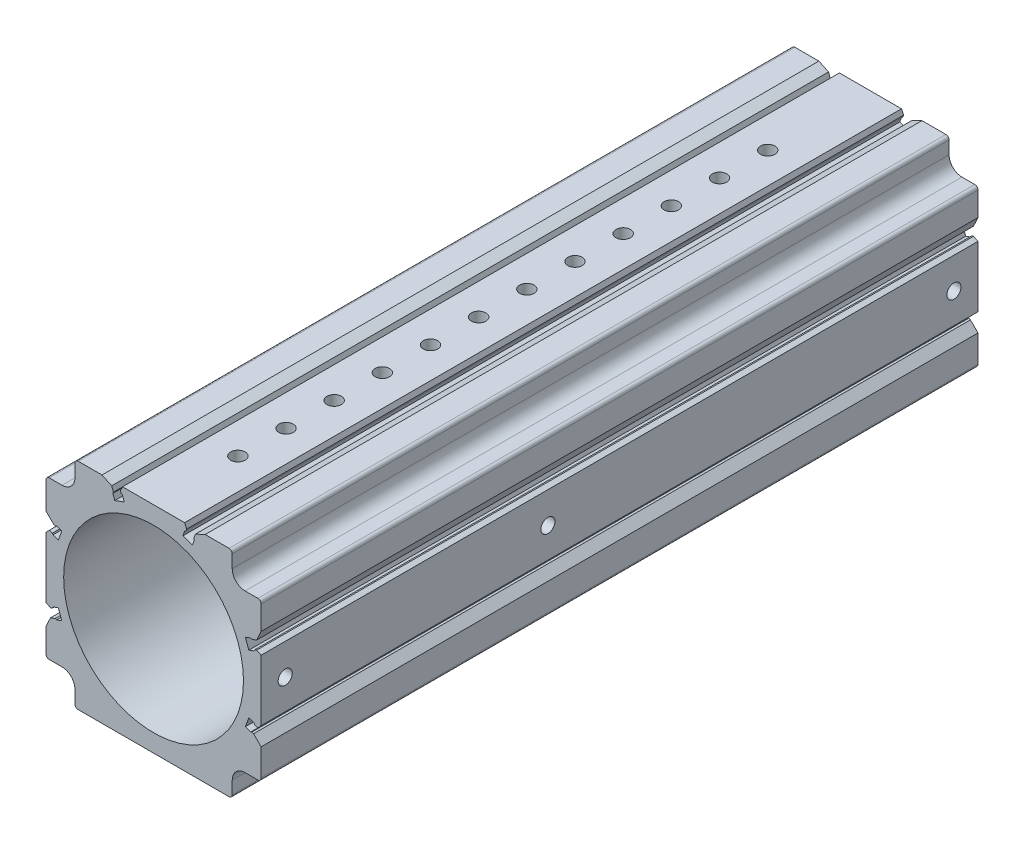
SolidWorks part; units mm, degrees
material "电镀钢"
ref_plane "Front Plane" through (0, 0, 0) normal (0, 0, 1) x (1, 0, 0)
ref_plane "Top Plane" through (0, 0, 0) normal (0, 1, 0) x (1, 0, 0)
ref_plane "Right Plane" through (0, 0, 0) normal (1, 0, 0) x (0, 0, -1)
sketch "Sketch1" plane through (0, 0, 0) normal (0, 0, 1) x (1, 0, 0)
  line L0 (-44.8, 67) -> (-36.9132, 67)
  line L1 (36.9132, 67) -> (44.8, 67)
  line L2 (67, 36.9132) -> (67, 44.8)
  line L3 (67, -44.8) -> (67, -36.9132)
  line L4 (-44.8, -67) -> (-36.9132, -67)
  line L5 (36.9132, -67) -> (44.8, -67)
  line L6 (-67, -44.8) -> (-67, -36.9132)
  line L7 (-67, 44.8) -> (-67, 36.9132)
  line L77 (67, -32.6) -> (67, -36.9132)
  line L79 (67, 27.5) -> (66.1, 27.5)
  line L80 (67, 57) -> (67, 44.8)
  line L81 (66.1, 32.6) -> (67, 32.6)
  line L82 (67, 27.5) -> (67, -27.5)
  line L83 (66.1, -27.5) -> (67, -27.5)
  line L84 (67, -32.6) -> (66.1, -32.6)
  line L85 (67, 36.9132) -> (67, 32.6)
  line L86 (65.5, -26.9) -> (62, -26.9)
  line L87 (62, 26.9) -> (65.5, 26.9)
  line L88 (62, -33.2) -> (65.5, -33.2)
  line L89 (65.5, 33.2) -> (62, 33.2)
  line L90 (62, -26.9) -> (62, -33.2)
  line L91 (62, 33.2) -> (62, 26.9)
  line L92 (57, -67) -> (44.8, -67)
  line L94 (67, -44.8) -> (67, -57)
  line L98 (44.8, 67) -> (57, 67)
  line L99 (32.6, 67) -> (36.9132, 67)
  line L100 (-36.9132, -67) -> (36.9132, -67)
  line L101 (33.2, 62) -> (33.2, 65.5)
  line L102 (26.9, 62) -> (33.2, 62)
  line L105 (32.6, 67) -> (32.6, 66.1)
  line L106 (27.5, 66.1) -> (27.5, 67)
  line L107 (-27.5, 67) -> (27.5, 67)
  line L108 (26.9, 65.5) -> (26.9, 62)
  line L109 (-33.2, 62) -> (-26.9, 62)
  line L110 (-26.9, 62) -> (-26.9, 65.5)
  line L111 (-27.5, 67) -> (-27.5, 66.1)
  line L112 (-36.9132, 67) -> (-32.6, 67)
  line L113 (-32.6, 66.1) -> (-32.6, 67)
  line L114 (-33.2, 65.5) -> (-33.2, 62)
  line L116 (-44.8, -67) -> (-57, -67)
  line L120 (-57, 67) -> (-44.8, 67)
  line L122 (-67, 32.6) -> (-67, 36.9132)
  line L123 (-62, 26.9) -> (-62, 33.2)
  line L124 (-65.5, 26.9) -> (-62, 26.9)
  line L125 (-62, 33.2) -> (-65.5, 33.2)
  line L126 (-62, -33.2) -> (-62, -26.9)
  line L127 (-62, -26.9) -> (-65.5, -26.9)
  line L128 (-65.5, -33.2) -> (-62, -33.2)
  line L130 (-67, 32.6) -> (-66.1, 32.6)
  line L131 (-67, -27.5) -> (-66.1, -27.5)
  line L132 (-66.1, 27.5) -> (-67, 27.5)
  line L133 (-66.1, -32.6) -> (-67, -32.6)
  line L134 (-67, -57) -> (-67, -44.8)
  line L135 (-67, -36.9132) -> (-67, -32.6)
  line L136 (-67, -27.5) -> (-67, 27.5)
  line L139 (-67, 44.8) -> (-67, 57)
  line L140 (-65.5, 33.2) -> (-66.1, 32.6)
  line L141 (-66.1, 27.5) -> (-65.5, 26.9)
  line L142 (-65.5, -26.9) -> (-66.1, -27.5)
  line L143 (-66.1, -32.6) -> (-65.5, -33.2)
  line L144 (65.5, -33.2) -> (66.1, -32.6)
  line L145 (66.1, -27.5) -> (65.5, -26.9)
  line L146 (65.5, 26.9) -> (66.1, 27.5)
  line L147 (66.1, 32.6) -> (65.5, 33.2)
  line L148 (33.2, 65.5) -> (32.6, 66.1)
  line L149 (27.5, 66.1) -> (26.9, 65.5)
  line L150 (-26.9, 65.5) -> (-27.5, 66.1)
  line L151 (-32.6, 66.1) -> (-33.2, 65.5)
  arc A15 (-67, -57) -> (-57, -67) centre (-57, -57) ccw
  arc A18 (57, -67) -> (67, -57) centre (57, -57) ccw
  arc A21 (67, 57) -> (57, 67) centre (57, 57) ccw
  arc A24 (-57, 67) -> (-67, 57) centre (-57, 57) ccw
  circle A25 centre (0, 0) radius 56
extrude "Boss-Extrude1" add sketch "Sketch1" along normal blind 446.5
sketch "Sketch3" plane through (0, 0, 446.5) normal (0, 0, 1) x (1, 0, 0)
  line L1 (-49, 49) -> (-73.0007, 49)
  line L2 (-49, 49) -> (-49, 80.3117)
  line L3 (-49, 80.3117) -> (-73.0007, 80.3117)
  line L4 (-73.0007, 49) -> (-73.0007, 80.3117)
  line L5 (-49, 49) -> (-73.0007, 80.3117) construction
  line L6 (-49, 80.3117) -> (-73.0007, 49) construction
  line L8 (-32.6, 67) -> (-57, 67) construction
  line L9 (-67, 57) -> (-67, 32.6) construction
  point P0 (-61.0004, 64.6558)
  dimension "D1" = 18
  dimension "D2" = 18
extrude "Cut-Extrude2" cut sketch "Sketch3" against normal through all
fillet "Fillet1" radius 8 1 edges at (-49, 49, 223.25)
pattern_circular "CirPattern1" count 4 over 360 about axis through (0, 0, 0) along (0, 0, 1) of "Cut-Extrude2", "Fillet1"
hole_wizard "Ø9.0 (9) Diameter Hole1" positions "Sketch6" profile "Sketch8" hole size "Ø9.0" standard "GB"
sketch "Sketch6" plane through (0, 67, 0) normal (0, -1, 0) x (-1, 0, 0)
  line L0 (0, 0) -> (0, -285.4047) construction
  line L4 (49, -446.5) -> (-49, -446.5) construction
  point P0 (0, -394)
  dimension "D1" = 52.5
sketch "Sketch8" plane through (0, 67, 394) normal (1, 0, 0) x (0, 0, 1)
  line L0 (0, 0) -> (0, 22.7039)
  line L1 (0, 22.7039) -> (4.5, 20)
  line L2 (4.5, 20) -> (4.5, 0)
  line L5 (4.5, 0) -> (0, 0)
  line L10 (0, 22.7039) -> (-4.5, 20) construction
  line L11 (0, -6.35) -> (0, 107.95) construction
  dimension "孔直径" = 9
  dimension "孔深度" = 20
  dimension "导头角度" = 118
hole_wizard "M12 Tapped Hole1" positions "Sketch9" profile "Sketch11" tap size "M12" standard "GB"
sketch "Sketch9" plane through (67, -134, 0) normal (-1, 0, 0) x (0, 0, -1)
  line L0 (0, -134) -> (-113.15, -134) construction
  line L4 (-411, -106.5) -> (-411, -161.5) construction
  point P2 (-394, -134)
  dimension "D1" = 17
sketch "Sketch11" plane through (67, 0, 394) normal (0, 1, 0) x (0, 0, -1)
  line L0 (0, 0) -> (0, 32.3144)
  line L1 (0, 32.3144) -> (5.1, 29.25)
  line L2 (5.1, 29.25) -> (5.1, 0)
  line L5 (5.1, 0) -> (0, 0)
  line L10 (0, 32.3144) -> (-5.1, 29.25) construction
  line L11 (0, -6.35) -> (0, 107.95) construction
  dimension "螺纹孔钻头直径" = 10.2
  dimension "螺纹孔钻头深度" = 29.25
  dimension "导头角度" = 118
cosmetic thread "Cosmetic thread 4" [suppressed] parameters "D1"=4.7084, "D2"=12
hole_wizard "M12 Tapped Hole2" positions "Sketch16" profile "Sketch17" tap size "M12" standard "GB"
sketch "Sketch16" plane through (67, 0, 0) normal (-1, 0, 0) x (0, 0, 1)
  point P0 (17, 0)
  dimension "D1" = 17
sketch "Sketch17" plane through (67, 0, 17) normal (0, 1, 0) x (0, 0, -1)
  line L0 (0, 0) -> (0, 32.3144)
  line L1 (0, 32.3144) -> (5.1, 29.25)
  line L2 (5.1, 29.25) -> (5.1, 0)
  line L5 (5.1, 0) -> (0, 0)
  line L10 (0, 32.3144) -> (-5.1, 29.25) construction
  line L11 (0, -6.35) -> (0, 107.95) construction
  dimension "螺纹孔钻头直径" = 10.2
  dimension "螺纹孔钻头深度" = 29.25
  dimension "导头角度" = 118
cosmetic thread "Cosmetic thread 5" [suppressed] parameters "D1"=4.7084, "D2"=12
pattern_linear "LPattern1" count 12 spacing 30 along (0, 0, -1) of "Ø9.0 (9) Diameter Hole1"
hole_wizard "G1/8 Tapped Hole1" positions "Sketch18" profile "Sketch19" tap size "G1/8" standard "GB"
sketch "Sketch18" plane through (67, 0, 0) normal (1, 0, 0) x (0, 0, -1)
  line L1 (0, -27.5) -> (0, 27.5) construction
  point P0 (-267.9, 0)
  dimension "D1" = 267.9
sketch "Sketch19" plane through (67, 0, 267.9) normal (0, 1, 0) x (0, 0, -1)
  line L0 (0, 0) -> (0, 24.8238)
  line L1 (0, 24.8238) -> (4.4, 22.18)
  line L2 (4.4, 22.18) -> (4.4, 0)
  line L5 (4.4, 0) -> (0, 0)
  line L10 (0, 24.8238) -> (-4.4, 22.18) construction
  line L11 (0, -6.35) -> (0, 107.95) construction
  dimension "螺纹孔钻头直径" = 8.8
  dimension "螺纹孔钻头深度" = 22.18
  dimension "导头角度" = 118
cosmetic thread "Cosmetic thread 9" parameters "D1"=4.6551, "D2"=9.728
fillet "Fillet2" radius 2 8 edges at (49, 67, 223.25) (67, 49, 223.25) (67, -49, 223.25) (49, -67, 223.25) (-49, -67, 223.25) (-67, -49, 223.25) (-67, 49, 223.25) (-49, 67, 223.25)
sketch "Sketch20" plane through (67, 0, 0) normal (1, 0, 0) x (0, 0, -1)
  line L0 (-431.5, 0) -> (-15, 0) construction
  line L1 (-446.5, -27.5) -> (-446.5, 27.5) construction
  line L2 (0, -27.5) -> (0, 27.5) construction
  circle A0 centre (-431.5, 0) radius 5
  circle A1 centre (-15, 0) radius 5
  dimension "D1" = 15
  dimension "D2" = 15
hole_wizard "G1/8 Tapped Hole2" positions "Sketch21" profile "Sketch22" tap size "G1/8" standard "GB"
sketch "Sketch21" plane through (67, 0, 0) normal (1, 0, 0) x (0, 0, -1)
  point P0 (-431.5, 0)
  point P3 (-15, 0)
sketch "Sketch22" plane through (67, 0, 431.5) normal (0, 1, 0) x (0, 0, -1)
  line L0 (0, 0) -> (0, 24.8238)
  line L1 (0, 24.8238) -> (4.4, 22.18)
  line L2 (4.4, 22.18) -> (4.4, 0)
  line L5 (4.4, 0) -> (0, 0)
  line L10 (0, 24.8238) -> (-4.4, 22.18) construction
  line L11 (0, -6.35) -> (0, 107.95) construction
  dimension "螺纹孔钻头直径" = 8.8
  dimension "螺纹孔钻头深度" = 22.18
  dimension "导头角度" = 118
cosmetic thread "Cosmetic thread 10" parameters "D1"=4.6551, "D2"=9.728
cosmetic thread "Cosmetic thread 11" parameters "D1"=4.6551, "D2"=9.728
sketch "Sketch23" plane through (0, 0, 0) normal (0, 0, -1) x (-1, 0, 0)
  line L0 (-23.1301, -51) -> (23.1301, -51)
  line L1 (47, -67) -> (-47, -67) construction
  circle A0 centre (0, 0) radius 56 construction
  arc A1 (-23.1301, -51) -> (23.1301, -51) centre (0, 0) ccw
  dimension "D1" = 16
extrude "Boss-Extrude2" [suppressed] add sketch "Sketch23" against normal through all
fillet "Fillet3" [suppressed] radius 10
other "Move Face1" [suppressed] parameters "D1"=6.5
sketch "Sketch24" plane through (0, 67, 0) normal (0, 1, 0) x (1, 0, 0)
  circle A0 centre (0, -394) radius 8
  dimension "D1" = 16
extrude "Cut-Extrude3" [suppressed] cut sketch "Sketch24" against normal blind 4
pattern_linear "LPattern2" [suppressed] count 7 spacing 30
sketch "Sketch25" plane through (0, 0, 446.5) normal (0, 0, 1) x (1, 0, 0)
  line L0 (0, 0) -> (0, 67) construction
  line L1 (27.5, 67) -> (-27.5, 67) construction
  line L2 (0, 0) -> (-25.07, 68.8793) construction
  line L3 (-18.2452, 59.3383) -> (-24.1653, 57.1836)
  line L4 (-24.1653, 57.1836) -> (-25.3624, 60.4725)
  line L5 (-18.2452, 59.3383) -> (-19.4423, 62.6272)
  line L6 (-25.3624, 60.4725) -> (-25.0037, 61.2415)
  line L7 (-25.0037, 61.2415) -> (-27.4907, 68.0745)
  line L8 (-19.4423, 62.6272) -> (-20.2113, 62.9858)
  line L9 (-20.2113, 62.9858) -> (-22.6983, 69.8188)
  line L10 (-22.6983, 69.8188) -> (-27.4907, 68.0745)
  circle A0 centre (0, 0) radius 56 construction
  dimension "D1" = 20
  dimension "D2" = 90
  dimension "D3" = 62
  dimension "D4" = 6.3
  dimension "D5" = 3.15
  dimension "D6" = 90
  dimension "D7" = 90
  dimension "D8" = 3.5
  dimension "D9" = 3.5
  dimension "D10" = 5.1
  dimension "D11" = 2.55
  dimension "D12" = 135
  dimension "D13" = 135
  dimension "D14" = 90
  dimension "D15" = 90
extrude "Cut-Extrude4" cut sketch "Sketch25" against normal through all
sketch "Sketch26" plane through (0, 0, 446.5) normal (0, 0, 1) x (1, 0, 0)
  line L0 (-27.5, 67) -> (-26.29, 64.4296)
  line L1 (-26.29, 64.4296) -> (-26.4603, 61.3407)
  line L2 (-26.4603, 61.3407) -> (-34.0001, 61.1462)
  line L3 (-34.0001, 61.1462) -> (-34.0001, 67)
  line L4 (-32.6, 67) -> (-47, 67) construction
  line L5 (-34.0001, 67) -> (-27.5, 67)
extrude "Boss-Extrude3" add sketch "Sketch26" against normal through all
chamfer "Chamfer2" distance 3 angle 45 1 edges at (-21.6724, 67, 223.25)
chamfer "Chamfer3" distance 3 angle 45 1 edges at (-27.0997, 67, 223.25)
mirror "Mirror1" about plane through (0, 0, 0) normal (1, 0, 0) of "Chamfer2", "Chamfer3", "Boss-Extrude3", "Cut-Extrude4"
pattern_circular "CirPattern13" count 4 over 360 about axis through (0, 0, 0) along (0, 0, 1) skipping 2 of "Cut-Extrude4"
pattern_circular "CirPattern14" count 4 over 360 about axis through (0, 0, 446.5) along (0, 0, -1) skipping 2 of "Boss-Extrude3"
mirror "Mirror2" about plane through (0, 0, 0) normal (0, 1, 0) of "CirPattern13", "Cut-Extrude4"
sketch "Sketch28" plane through (0, 0, 446.5) normal (0, 0, 1) x (1, 0, 0)
  line L0 (-27.0997, -67) -> (-21.6724, -67)
  line L1 (-21.6724, -67) -> (-15.1959, -57.9166)
  line L2 (-15.1959, -57.9166) -> (-28.9583, -52.9469)
  line L3 (-28.9583, -52.9469) -> (-27.0997, -67)
  line L4 (-67, 27.5) -> (-67, 32.6)
  line L5 (-67, 32.6) -> (-62.0056, 35.1671)
  line L6 (-62.0056, 35.1671) -> (-60.0646, 33.1648)
  line L7 (-60.0646, 33.1648) -> (-60.7664, 26.6143)
  line L8 (-60.7664, 26.6143) -> (-64.0283, 26.6143)
  line L9 (-64.0283, 26.6143) -> (-65.6774, 26.791)
  line L10 (-65.6774, 26.791) -> (-67, 27.5)
  line L11 (67, -27.5) -> (67, -32.6)
  line L12 (67, -32.6) -> (64.4183, -34.1929)
  line L13 (64.4183, -34.1929) -> (60.8641, -33.8121)
  line L14 (60.8641, -33.8121) -> (60.6405, -29.2349)
  line L15 (60.6405, -29.2349) -> (60.9192, -26.6336)
  line L16 (60.9192, -26.6336) -> (64.7514, -26.4463)
  line L17 (64.7514, -26.4463) -> (66.1689, -27.0788)
  line L18 (66.1689, -27.0788) -> (67, -27.5)
extrude "Boss-Extrude4" add sketch "Sketch28" against normal through all contours L3 L0 L1 L2 | L18 L11 L12 L13 L14 L15 L16 L17 | L10 L4 L5 L6 L7 L8 L9
chamfer "Chamfer4" distance 3 angle 45 8 edges at (-67, -21.6724, 223.25) (-67, -27.0997, 223.25) (67, 21.6724, 223.25) (67, 27.0997, 223.25) (-67, 27.0997, 223.25) (-67, 21.6724, 223.25) (67, -27.0997, 223.25) (67, -21.6724, 223.25)
